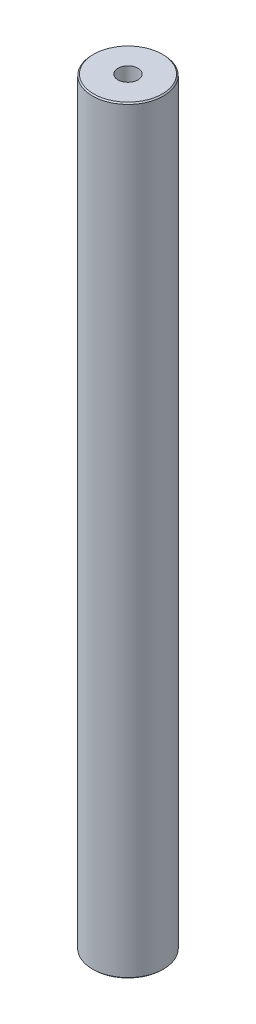
from build123d import *

# Parameters (mm, degrees)
SKETCH_1_R              = 15
EXTRUDE_1_DEPTH         = 160
CHAMFER_1_SIZE          = 0.5
HOLE_WIZARD_M10_2_D     = 8.5
HOLE_WIZARD_M10_2_DEPTH = 24.5
HOLE_WIZARD_M10_2_TIP   = 2.553657631
HOLE_WIZARD_M10_1_D     = 8.5
HOLE_WIZARD_M10_1_DEPTH = 24.5
HOLE_WIZARD_M10_1_TIP   = 2.553657631


with BuildPart() as part:
    # 草图1 → 凸台-拉伸1 (new, symmetric)
    with BuildSketch(Plane(origin=(0, 0, 0), x_dir=(1, 0, 0), z_dir=(0, 1, 0))):
        with Locations(Location((0, 0, 0), (0, 0, 270))):
            Circle(SKETCH_1_R)
    extrude(amount=EXTRUDE_1_DEPTH, both=True)

    # 倒角1
    chamfer_1_edges = [part.edges().sort_by_distance(p)[0] for p in [
        (0, -160, -15),
        (0, 160, -15),
    ]]
    chamfer(chamfer_1_edges, length=CHAMFER_1_SIZE)

    # M10 螺纹孔2
    with Locations(Plane(origin=(0, 160, 0), x_dir=(1, 0, 0), z_dir=(0, 1, 0))):
        with Locations((0, 0)):
            Hole(HOLE_WIZARD_M10_2_D / 2, depth=HOLE_WIZARD_M10_2_DEPTH)
            with Locations((0, 0, -(HOLE_WIZARD_M10_2_DEPTH + HOLE_WIZARD_M10_2_TIP / 2))):  # 118° drill point
                Cone(0, HOLE_WIZARD_M10_2_D / 2, HOLE_WIZARD_M10_2_TIP, mode=Mode.SUBTRACT)

    # M10 螺纹孔1
    with Locations(Plane(origin=(0, -160, 0), x_dir=(-1, 0, 0), z_dir=(0, -1, 0))):
        with Locations((0, 0)):
            Hole(HOLE_WIZARD_M10_1_D / 2, depth=HOLE_WIZARD_M10_1_DEPTH)
            with Locations((0, 0, -(HOLE_WIZARD_M10_1_DEPTH + HOLE_WIZARD_M10_1_TIP / 2))):  # 118° drill point
                Cone(0, HOLE_WIZARD_M10_1_D / 2, HOLE_WIZARD_M10_1_TIP, mode=Mode.SUBTRACT)


solid = part.part
